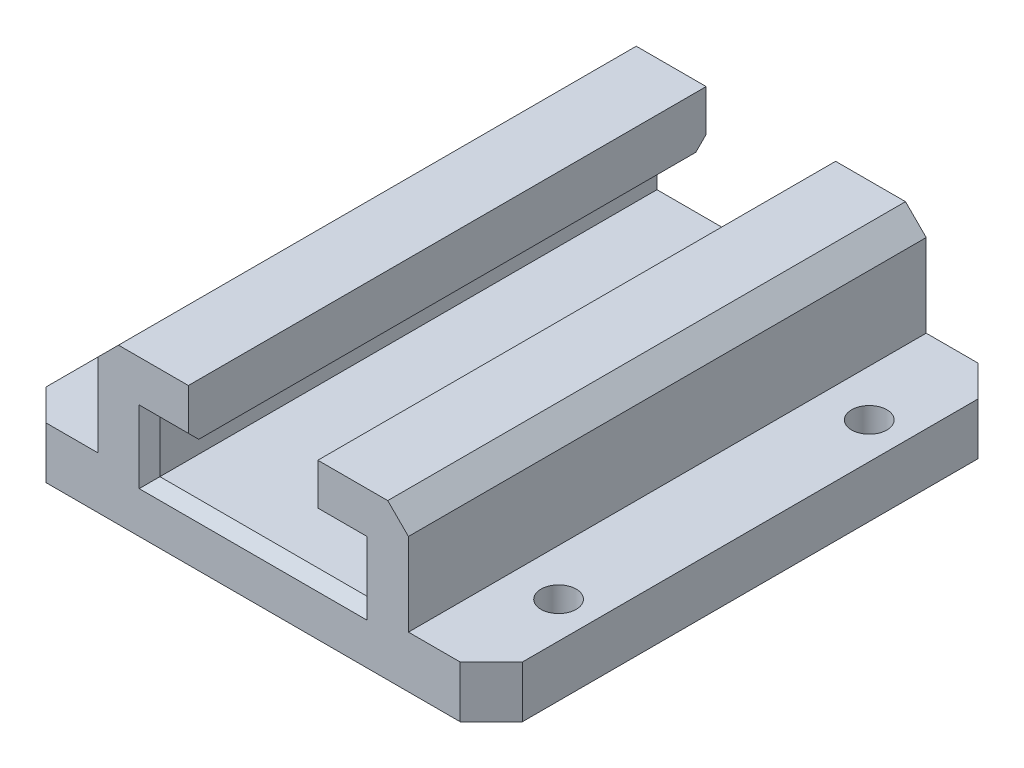
from build123d import *

# Parameters (mm, degrees)
EXTRUDE_1_DEPTH    = 50
SKETCH_3_W         = 8
SKETCH_3_H         = 5
EXTRUDE_2_DEPTH    = 50
CHAMFER_1_SIZE     = 1
CHAMFER_2_SIZE     = 1
CHAMFER_3_SIZE     = 3
HOLE_WIZARD_M3_1_D = 3.4
CHAMFER_4_SIZE     = 2


with BuildPart() as part:
    # 草图1 → 凸台-拉伸1 (new body)
    with BuildSketch(Plane.XY):
        Polygon((15, 0), (-15, 0), (-15, 15), (-6.25, 15), (-6.25, 10), (-10, 10), (-10, 5), (10, 5), (10, 10), (6.25, 10), (6.25, 15), (15, 15), align=None)
    extrude(amount=EXTRUDE_1_DEPTH)

    # 草图3 → 凸台-拉伸2 (add)
    with BuildSketch(Plane.XY.offset(50)):
        with Locations((-19, 2.5)):
            Rectangle(SKETCH_3_W, SKETCH_3_H)
        with Locations((19, 2.5)):
            Rectangle(SKETCH_3_W, SKETCH_3_H)
    extrude(amount=-EXTRUDE_2_DEPTH)

    # 倒角1
    chamfer_1_edges = [part.edges().sort_by_distance(p)[0] for p in [
        (8.125, 10, 50),
        (10, 7.5, 50),
        (0, 5, 50),
        (-10, 7.5, 50),
        (-8.125, 10, 50),
    ]]
    chamfer(chamfer_1_edges, length=CHAMFER_1_SIZE)

    # 倒角2
    chamfer_2_edges = [part.edges().sort_by_distance(p)[0] for p in [
        (-8.125, 10, 0),
        (-10, 7.5, 0),
        (0, 5, 0),
        (10, 7.5, 0),
        (8.125, 10, 0),
    ]]
    chamfer(chamfer_2_edges, length=CHAMFER_2_SIZE)

    # 倒角3
    chamfer_3_edges = [part.edges().sort_by_distance(p)[0] for p in [
        (-23, 2.5, 50),
        (-23, 2.5, 0),
        (23, 2.5, 50),
        (23, 2.5, 0),
    ]]
    chamfer(chamfer_3_edges, length=CHAMFER_3_SIZE)

    # M3 间隙孔1 (through all)
    with Locations(Plane(origin=(0, 5, 0), x_dir=(1, 0, 0), z_dir=(0, 1, 0))):
        with Locations((-19.5, -10), (-19.5, -40), (19.5, -40), (19.5, -10)):
            Hole(HOLE_WIZARD_M3_1_D / 2)

    # 倒角4
    chamfer_4_edges = [part.edges().sort_by_distance(p)[0] for p in [
        (-15, 15, 25),
        (15, 15, 25),
    ]]
    chamfer(chamfer_4_edges, length=CHAMFER_4_SIZE)


solid = part.part
